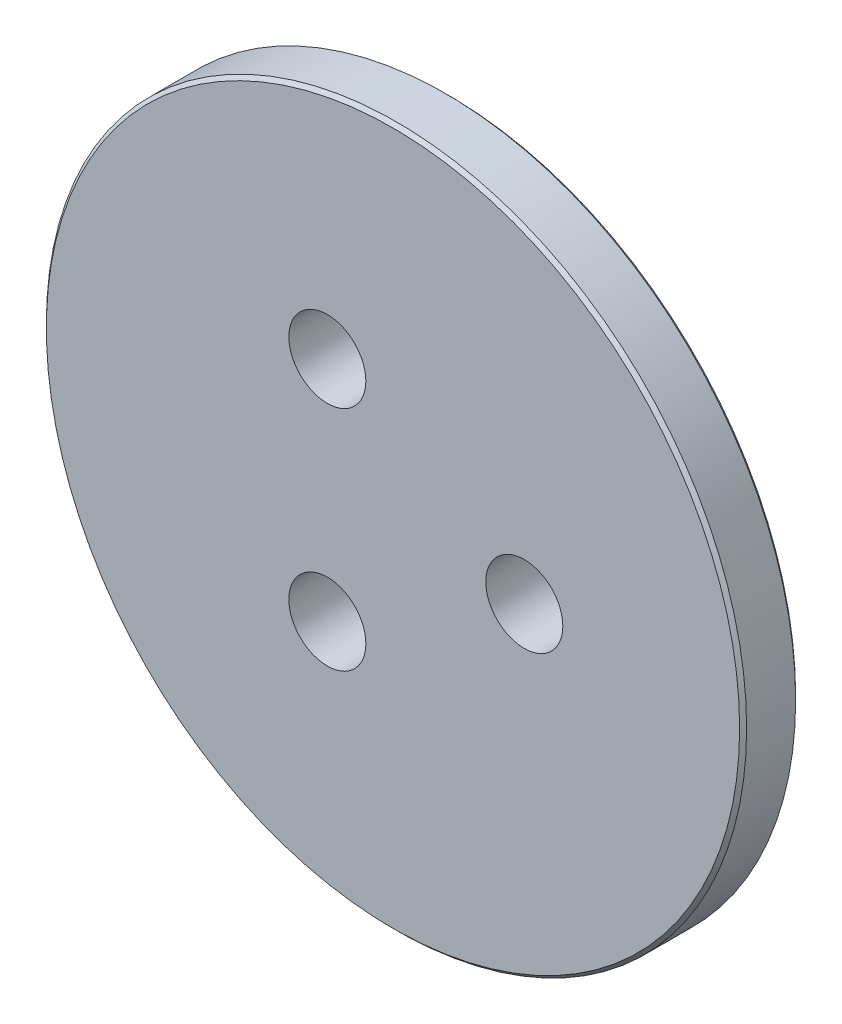
SolidWorks part; units mm, degrees
material "Plain Carbon Steel"
ref_plane "Front Plane" through (0, 0, 0) normal (0, 0, 1) x (1, 0, 0)
ref_plane "Top Plane" through (0, 0, 0) normal (0, 1, 0) x (1, 0, 0)
ref_plane "Right Plane" through (0, 0, 0) normal (1, 0, 0) x (0, 0, -1)
sketch "Sketch1" plane through (0, 0, 0) normal (0, 0, 1) x (1, 0, 0)
  circle A0 centre (0, 0) radius 100
  dimension "D1" = 200
extrude "Boss-Extrude1" add sketch "Sketch1" along normal blind 16
sketch "Sketch2" plane through (0, 0, 16) normal (0, 0, 1) x (1, 0, 0)
  circle A0 centre (0, 0) radius 37.5 construction
  circle A1 centre (37.5, 0) radius 11
  dimension "D1" = 75
  dimension "D2" = 22
extrude "Cut-Extrude1" cut sketch "Sketch2" against normal through all
pattern_circular "CirPattern1" count 3 over 360 about axis through (0, 0, 0) along (0, 0, 1) of "Cut-Extrude1"
chamfer "Chamfer1" distance 1 angle 45 2 edges at (100, 0, 0) (100, 0, 16)
